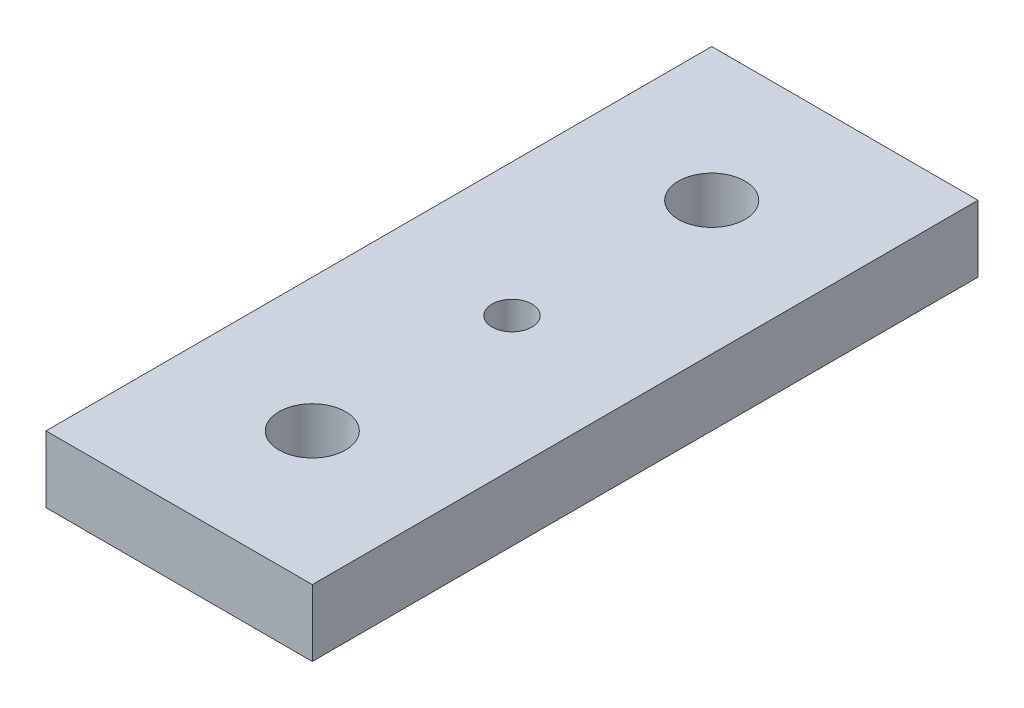
SolidWorks part; units mm, degrees
ref_plane "Front Plane" through (0, 0, 0) normal (0, 0, 1) x (1, 0, 0)
ref_plane "Top Plane" through (0, 0, 0) normal (0, 1, 0) x (1, 0, 0)
ref_plane "Right Plane" through (0, 0, 0) normal (1, 0, 0) x (0, 0, -1)
sketch "Sketch1" plane through (0, 0, 0) normal (0, 1, 0) x (1, 0, 0)
  line L1 (20, 50) -> (-20, 50)
  line L2 (20, 50) -> (20, -50)
  line L3 (20, -50) -> (-20, -50)
  line L4 (-20, 50) -> (-20, -50)
  line L5 (20, 50) -> (-20, -50) construction
  line L6 (20, -50) -> (-20, 50) construction
  circle A0 centre (0, 0) radius 3
  circle A1 centre (0, -30) radius 5
  circle A2 centre (0, 30) radius 5
  point P0 (0, 0)
  dimension "D3" = 6
  dimension "D6" = 10
  dimension "D7" = 10
  dimension "D1" = 100
  dimension "D2" = 40
  dimension "D4" = 30
  dimension "D5" = 30
extrude "Boss-Extrude1" add sketch "Sketch1" along normal blind 10 contours L1 L4 L3 L2 A2 A1 A0
